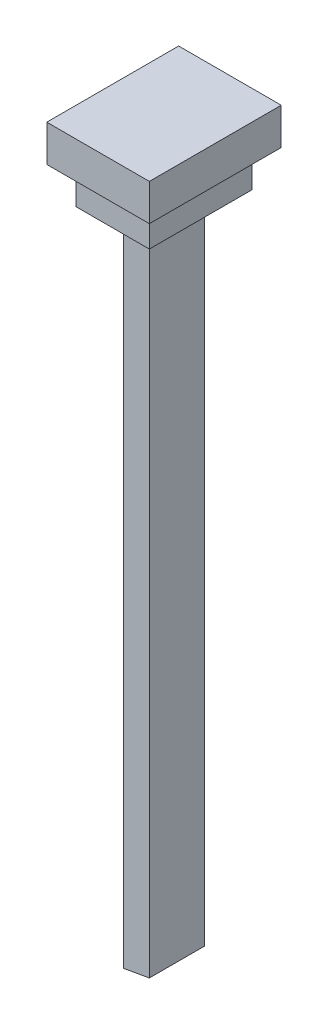
SolidWorks part; units mm, degrees
ref_plane "Front Plane" through (0, 0, 0) normal (0, 0, 1) x (1, 0, 0)
ref_plane "Top Plane" through (0, 0, 0) normal (0, 1, 0) x (1, 0, 0)
ref_plane "Right Plane" through (0, 0, 0) normal (1, 0, 0) x (0, 0, -1)
sketch "Sketch1" plane through (0, 0, 0) normal (0, 1, 0) x (1, 0, 0)
  line L4 (0, 0) -> (0, 4.2941) construction
  line L5 (0, 0) -> (3.6898, 0) construction
  line L6 (-0.89, 1.89) -> (0.89, 1.89)
  line L7 (0.89, 1.89) -> (0.89, -1.89)
  line L8 (0.89, -1.89) -> (-0.89, -1.89)
  line L9 (-0.89, -1.89) -> (-0.89, 1.89)
extrude "Boss-Extrude1" add sketch "Sketch1" along normal blind 45
sketch "Sketch2" plane through (0, 0, 1.89) normal (0, 0, 1) x (1, 0, 0)
  line L0 (-0.89, 0) -> (0.89, 0)
  line L1 (0.89, 0) -> (0.89, 0.3139)
  line L3 (0.89, 45) -> (0.89, 0) construction
  line L4 (0.89, 0.3139) -> (-0.89, 0)
  dimension "D1" = 10
extrude "Cut-Extrude1" cut sketch "Sketch2" against normal through all
sketch "Sketch3" plane through (0, 45, 0) normal (0, 1, 0) x (1, 0, 0)
  line L0 (-2.5, 3.5) -> (2.5, 3.5)
  line L5 (2.5, 3.5) -> (2.5, -3.5)
  line L6 (-2.5, -3.5) -> (2.5, -3.5)
  line L7 (-2.5, 3.5) -> (-2.5, -3.5)
extrude "Boss-Extrude2" add sketch "Sketch3" along normal blind 2.5
sketch "Sketch4" plane through (0, 47.5, 0) normal (0, 1, 0) x (1, 0, 0)
  line L0 (-3.5, 4.5) -> (3.5, 4.5)
  line L5 (3.5, 4.5) -> (3.5, -4.5)
  line L6 (-3.5, -4.5) -> (3.5, -4.5)
  line L7 (-3.5, 4.5) -> (-3.5, -4.5)
extrude "Boss-Extrude3" add sketch "Sketch4" along normal blind 2.5
